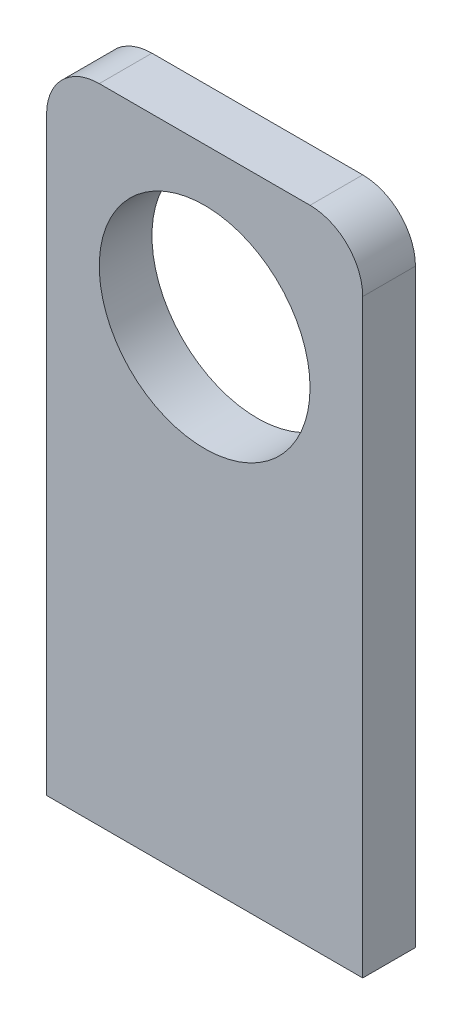
SolidWorks part; units mm, degrees
ref_plane "前视基准面" through (0, 0, 0) normal (0, 0, 1) x (1, 0, 0)
ref_plane "上视基准面" through (0, 0, 0) normal (0, 1, 0) x (1, 0, 0)
ref_plane "右视基准面" through (0, 0, 0) normal (1, 0, 0) x (0, 0, -1)
sketch "草图1" plane through (0, 0, 0) normal (0, 0, 1) x (1, 0, 0)
  line L1 (-15, -30.5) -> (15, -30.5)
  line L2 (-15, -30.5) -> (-15, 30.5)
  line L3 (-15, 30.5) -> (15, 30.5)
  line L4 (15, -30.5) -> (15, 30.5)
  line L5 (-15, -30.5) -> (15, 30.5) construction
  line L6 (-15, 30.5) -> (15, -30.5) construction
  circle A0 centre (0, 15.5) radius 10
  point P0 (0, 0)
  point P8 (0, 0)
  dimension "D3" = 20
  dimension "D1" = 30
  dimension "D2" = 61
  dimension "D4" = 15
extrude "凸台-拉伸1" add sketch "草图1" along normal mid plane 5
fillet "圆角1" radius 5 2 edges at (15, 30.5, 0) (-15, 30.5, 0)
